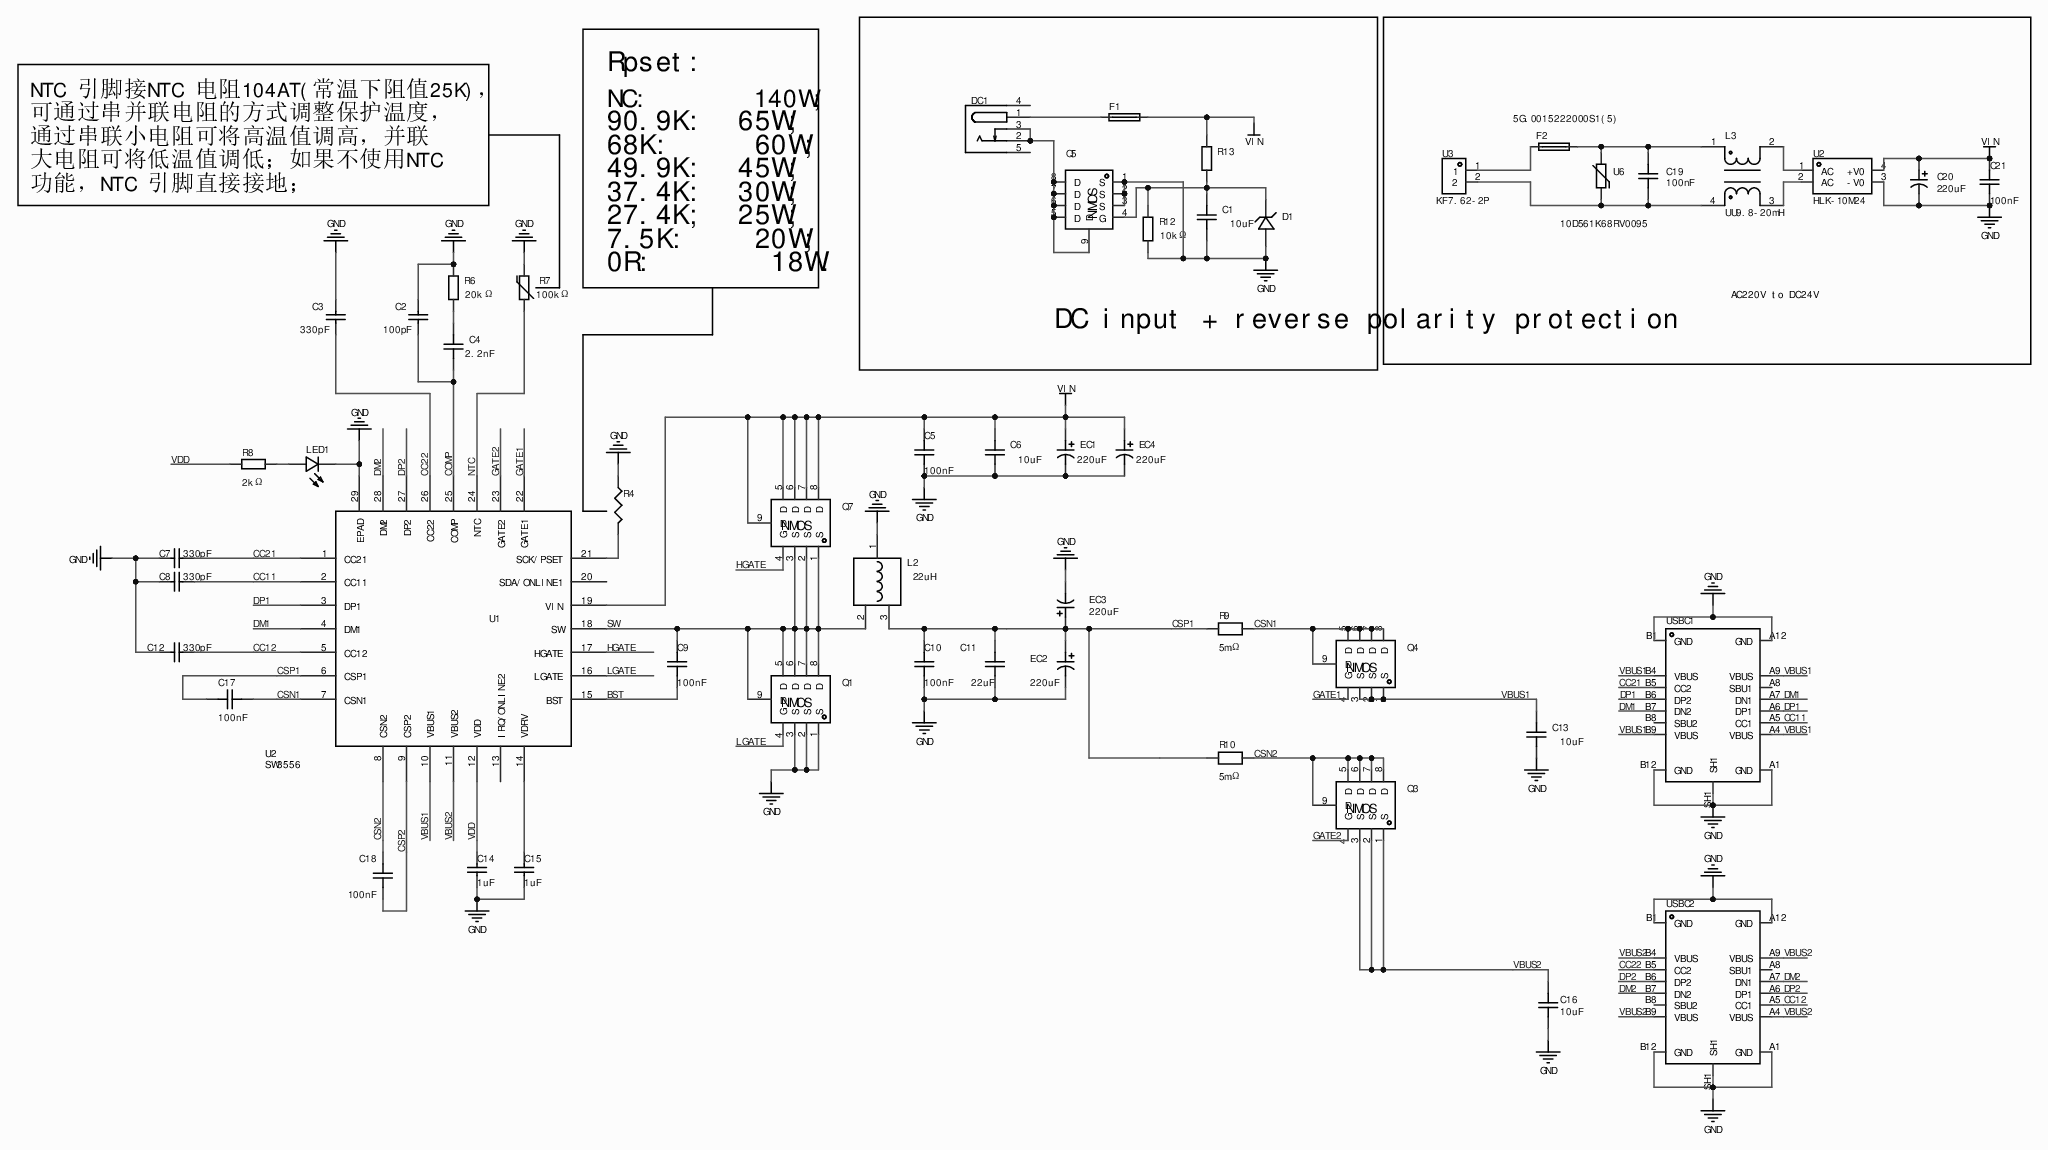
[diagram p0: MISC82101-2.schdoc]
# Altium project MISC82101-8.PrjPcb
1 sheet, 51 parts. Net scope: global (net labels, ports and power ports of the same name join across sheets).
Board file: MISC82101.pcbdoc

## Sheet MISC82101-2.schdoc
size 614 x 444 mm; @Project Name: MISC82101; @Page Count: 1; @Update Date: 2024-04-24; @Create Date: 2024-04-24; @Schematic Name: MISC82101; @Page No: 1

### Parts
C1  10uF  [C0805]
C2  100pF  [C0603]
C3  330pF  [C0603]
C4  2.2nF  [C0603]
C5  100nF  [C0603]
C6  10uF  [C0805]
C7  330pF  [C0603]
C8  330pF  [C0603]
C9  100nF  [C0603]
C10  100nF  [C0603]
C11  22uF  [C0805]
C12  330pF  [C0603]
C13  10uF  [C0805]
C14  1uF  [C0603]
C15  1uF  [C0603]
C16  10uF  [C0805]
C17  100nF  [C0603]
C18  100nF  [C0603]
C19  100nF  [CAP-TH_L13.0-W6.0-P10.0-D0.6]
C20  220uF  [CAP-TH_BD8.0-P3.50-D0.6-FD]
C21  100nF  [C0603]
D1  BZT52C3V3  [SOD-123_L2.7-W1.6-LS3.7-RD]  (value not drawn)
DC1  DC-044A-20A  [DC-IN-TH_DC-044A-20A]  (value not drawn)
EC1  220uF  [CAP-TH_BD8.0-P3.50-D0.6-FD-2]
EC2  220uF  [CAP-TH_BD8.0-P3.50-D0.6-FD-2]
EC3  220uF  [CAP-TH_BD8.0-P3.50-D0.6-FD-2]
EC4  220uF  [CAP-TH_BD8.0-P3.50-D0.6-FD-2]
F1  0451008.MRL  [FUSE-SMD_L6.1-W2.7]  (value not drawn)
F2  5G.0015222000S1(5)  [FUSE-TH_BD5.6-L21.0-P25.00-D0.7]
L2  22uH  [IND-SMD_3P-L15.5-W15.5-L]
L3  UU9.8-20mH  [FILTER-TH_4P-L17.0-W12.0-P7.00-D0.6-S8.00]
LED1  19-217/BHC-ZL1M2RY/3T  [LED0603-R-RD]  (value not drawn)
Q1  RUH4040M2  [PDFN3333-8_L3.1-W3.2-P0.65-LS3.4-BL]  (value not drawn)
Q3  RUH4040M2  [PDFN3333-8_L3.1-W3.2-P0.65-LS3.4-BL]  (value not drawn)
Q4  RUH4040M2  [PDFN3333-8_L3.1-W3.2-P0.65-LS3.4-BL]  (value not drawn)
Q5  RUH4040M2  [PDFN3333-8_L3.1-W3.2-P0.65-LS3.4-BL]  (value not drawn)
Q7  RUH4040M2  [PDFN3333-8_L3.1-W3.2-P0.65-LS3.4-BL]  (value not drawn)
R4  Rpset  [R0603]  (value not drawn)
R6  20kΩ  [R0603]
R7  Resistance @ 25℃: 100kΩ  [R0603]  (hidden comment: SDNT1608X104F4250FTF)
R8  value 2kΩ  [R0603]  (hidden comment: 0603WAF2001T5E)
R9  value 5mΩ  [R2010]  (hidden comment: RLM20FECR005)
R10  value 5mΩ  [R2010]  (hidden comment: RLM20FECR005)
R12  10kΩ  [R0603]
R13  0603WAF5102T5E  [R0603]  (value not drawn)
U1  sw3556-1  [QFN-28_L4.0-W4.0-P0.40-BL-EP]  (value not drawn)
U2  HLK-10M24  [PWRM-TH_HLK-10M24]
U3  KF7.62-2P  [CONN-TH_KF7.62-2P]
U6  10D561K68RV0095  [RES-TH_L13.5-W7.0-P7.50-S4.00-D0.7]
USBC1  U263-163N-4OS1735  [USB-C-SMD_U263-163N-4GS1735]  (value not drawn)
USBC2  U263-163N-4OS1735  [USB-C-SMD_U263-163N-4GS1735]  (value not drawn)

### Blocks framed on the sheet
DC input + reverse polarity protection: C1 D1 DC1 F1 Q5 R12 R13
AC220V to DC24V: C19-C21 F2 L3 U2 U3 U6

### Nets
GND: C1.1 C2.2 C3.2 C5.2 C6.1 C7.2 C8.2 C10.2 C11.1 C12.2 C13.1 C14.1 C15.1 C16.1 C20.2 C21.2 D1.2 EC1.2 EC2.2 EC3.2 EC4.2 L2.1 LED1.2(C) Q1.1(S) Q1.2(S) Q1.3(S) Q5.1(S) Q5.2(S) Q5.3(S) R4.1 R6.2 R7.1 R12.1 U1.29(EPAD) U2.3(-V0) USBC1.A1(GND) USBC1.A12(GND) USBC1.B1(GND) USBC1.B12(GND) USBC1.SH1 USBC2.A1(GND) USBC2.A12(GND) USBC2.B1(GND) USBC2.B12(GND) USBC2.SH1
VIN: C5.1 C6.2 C20.1 C21.1 EC1.1 EC4.1 F1.2 Q7.5(D) Q7.6(D) Q7.7(D) Q7.8(D) Q7.9(D) R13.2 U1.19(VIN) U2.4(+V0)
BST: C9.2 U1.15(BST)
CC11: C8.1 U1.2(CC11) USBC1.A5(CC1)
CC12: C12.1 U1.5(CC12) USBC2.A5(CC1)
CC21: C7.1 U1.1(CC21) USBC1.B5(CC2)
CC22: C3.1 U1.26(CC22) USBC2.B5(CC2)
COMP: C2.1 C4.1 U1.25(COMP)
CSN1: C17.1 Q4.5(D) Q4.6(D) Q4.7(D) Q4.8(D) Q4.9(D) R9.2 U1.7(CSN1)
CSN2: C18.1 Q3.5(D) Q3.6(D) Q3.7(D) Q3.8(D) Q3.9(D) R10.2 U1.8(CSN2)
CSP1: C10.1 C11.2 C17.2 C18.2 EC2.1 EC3.1 L2.3 R9.1 R10.1 U1.6(CSP1) U1.9(CSP2)  [also labelled CSP2, VOUT]
DM1: U1.4(DM1) USBC1.A7(DN1) USBC1.B7(DN2)
DM2: U1.28(DM2) USBC2.A7(DN1) USBC2.B7(DN2)
DP1: U1.3(DP1) USBC1.A6(DP1) USBC1.B6(DP2)
DP2: U1.27(DP2) USBC2.A6(DP1) USBC2.B6(DP2)
GATE1: Q4.4(G) U1.22(GATE1)
GATE2: Q3.4(G) U1.23(GATE2)
HGATE: Q7.4(G) U1.17(HGATE)
LGATE: Q1.4(G) U1.16(LGATE)
NTC: R7.2 U1.24(NTC)
SW: C9.1 L2.2 Q1.5(D) Q1.6(D) Q1.7(D) Q1.8(D) Q1.9(D) Q7.1(S) Q7.2(S) Q7.3(S) U1.18(SW)
VBUS1: C13.2 Q4.1(S) Q4.2(S) Q4.3(S) U1.10(VBUS1) USBC1.A4(VBUS) USBC1.A9(VBUS) USBC1.B4(VBUS) USBC1.B9(VBUS)
VBUS2: C16.2 Q3.1(S) Q3.2(S) Q3.3(S) U1.11(VBUS2) USBC2.A4(VBUS) USBC2.A9(VBUS) USBC2.B4(VBUS) USBC2.B9(VBUS)
VDD: C14.2 R8.1 U1.12(VDD)
NetC1_2: C1.2 D1.1 Q5.4(G) R12.2 R13.1
NetC4_2: C4.2 R6.1
NetC15_2: C15.2 U1.14(VDRV)
NetC19_1: C19.1 L3.4 U3.2 U6.1
NetC19_2: C19.2 F2.2 L3.1 U6.2
NetDC1_1: DC1.1 F1.1
NetDC1_2: DC1.2 DC1.3 Q5.5(D) Q5.6(D) Q5.7(D) Q5.8(D) Q5.9(D)
NetF2_1: F2.1 U3.1
NetL3_2: L3.2 U2.1(AC)
NetL3_3: L3.3 U2.2(AC)
NetLED1_1: LED1.1(A) R8.2
NetR4_2: R4.2 U1.21(SCK/PSET)

Not connected (* = marked no-connect by the designer): DC1 4* 5*; U1 13(IRQ/ONLINE2)* 20(SDA/ONLINE1)*; USBC1 A8(SBU1)* B8(SBU2)*; USBC2 A8(SBU1)* B8(SBU2)*

### Notes on the sheet
- Rpset:
- NC:       140W;
- 90.9K:  65W;
- 68K:     60W;
- 49.9K:  45W;
- NTC 引脚接NTC 电阻104AT(常温下阻值25K)，
  可通过串并联电阻的方式调整保护温度，
  通过串联小电阻可将高温值调高，并联
  大电阻可将低温值调低；如果不使用NTC
  功能，NTC 引脚直接接地；
- 37.4K:  30W;
- 27.4K;  25W;
- 7.5K:    20W;
- 0R:       18W.
- 1
- A

### Library data of the parts
C1 C6 C13 C16 = 10uF: Capacitance: 10uF; tolerance: ±10%; rated voltage: 50V; dielectric (temperature coefficient): X5R;; Manufacturer: muRata(村田); Symbol: GRM21BR61H106KE43L; Add into BOM: yes; Name: 10uF; Device: 10uF; LCSC Part Name: 10uF ±10% 50V; Supplier Part: C440198; Manufacturer Part: GRM21BR61H106KE43L; Supplier Footprint: 0805; JLCPCB Part Class: Basic library; Datasheet: https://atta.szlcsc.com/upload/public/pdf/source/20191220/C440198_2DEA1B9834E321C8893F7972E9DFE5B0.pdf; Supplier: LCSC; Convert to PCB: yes; Value: 10uF; Tolerance: ±10%; Voltage Rated: 50V; Temperature Coefficient: X5R; Origin Footprint 2: C0805; Origin Footprint 1: GRM21BR61H106KE43L
C2 = 100pF: Capacitance: 100pF; tolerance: ±5%; rated voltage: 50V; dielectric (temperature coefficient): C0G;; Manufacturer: SAMSUNG(三星); Symbol: CL10C101JB8NNNC; Add into BOM: yes; Name: 100pF; Device: 100pF; LCSC Part Name: 100pF ±5% 50V; Supplier Part: C14858; Manufacturer Part: CL10C101JB8NNNC; Supplier Footprint: 0603; JLCPCB Part Class: Basic library; Datasheet: https://atta.szlcsc.com/upload/public/pdf/source/20160103/1457707672333.pdf; Supplier: LCSC; Convert to PCB: yes; Value: 100pF; Tolerance: ±5%; Voltage Rated: 50V; Temperature Coefficient: C0G; Origin Footprint 2: C0603; Origin Footprint 1: CL10C101JB8NNNC
C3 C7 C8 C12 = 330pF: Capacitance: 330pF; tolerance: ±5%; rated voltage: 50V; dielectric (temperature coefficient): C0G;; Manufacturer: SAMSUNG(三星); Symbol: CL10C331JB8NNNC; Add into BOM: yes; Name: 330pF; Device: 330pF; LCSC Part Name: 330pF ±5% 50V; Supplier Part: C1664; Manufacturer Part: CL10C331JB8NNNC; Supplier Footprint: 0603; JLCPCB Part Class: Basic library; Datasheet: https://atta.szlcsc.com/upload/public/pdf/source/20160103/1457707688612.pdf; Supplier: LCSC; Convert to PCB: yes; Value: 330pF; Tolerance: ±5%; Voltage Rated: 50V; Temperature Coefficient: C0G; Origin Footprint 2: C0603; Origin Footprint 1: CL10C331JB8NNNC
C4 = 2.2nF: Capacitance: 2.2nF; tolerance: ±1%; rated voltage: -; dielectric (temperature coefficient): -;; Manufacturer: muRata(村田); Symbol: GCM1885C1H222FA16D; Add into BOM: yes; Name: 2.2nF; Device: 2.2nF; LCSC Part Name: 2.2nF ±1%; Supplier Part: C882578; Manufacturer Part: GCM1885C1H222FA16D; Supplier Footprint: 0603; JLCPCB Part Class: Extended library; Datasheet: https://atta.szlcsc.com/upload/public/pdf/source/20201228/C882578_EDF992AD6064A2D085B371C371799E69.pdf; Supplier: LCSC; Convert to PCB: yes; Value: 2.2nF; Tolerance: ±1%; Voltage Rated: -; Temperature Coefficient: -; Origin Footprint 2: C0603; Origin Footprint 1: GCM1885C1H222FA16D
C5 C9 C10 C17 C18 C21 = 100nF: Capacitance: 100nF; tolerance: ±10%; rated voltage: 50V; dielectric (temperature coefficient): X7R;; Manufacturer: YAGEO(国巨); Symbol: CC0603KRX7R9BB104; Add into BOM: yes; Name: 100nF; Device: 100nF; LCSC Part Name: 100nF ±10% 50V; Supplier Part: C14663; Manufacturer Part: CC0603KRX7R9BB104; Supplier Footprint: 0603; JLCPCB Part Class: Basic library; Datasheet: https://atta.szlcsc.com/upload/public/pdf/source/20170116/1484561234239.pdf; Supplier: LCSC; Convert to PCB: yes; Value: 100nF; Tolerance: ±10%; Voltage Rated: 50V; Temperature Coefficient: X7R; Origin Footprint 2: C0603; Origin Footprint 1: CC0603KRX7R9BB104
C11 = 22uF: Capacitance: 22uF; tolerance: ±20%; rated voltage: 25V; dielectric (temperature coefficient): X5R;; Manufacturer: SAMSUNG(三星); Manufacturer Part: CL21A226MAQNNNE; Symbol: CL21A226MAQNNNE_C45783; Add into BOM: yes; Name: 22uF; Device: 22uF; LCSC Part Name: 22uF ±20% 25V; Supplier Part: C45783; Supplier Footprint: 0805; JLCPCB Part Class: Basic library; Datasheet: https://atta.szlcsc.com/upload/public/pdf/source/20160103/1457707727161.pdf; Supplier: LCSC; Convert to PCB: yes; Value: 22uF; Tolerance: ±20%; Voltage Rated: 25V; Temperature Coefficient: X5R; Origin Footprint 2: C0805; Origin Footprint 1: CL21A226MAQNNNE_C45783
C14 C15 = 1uF: Capacitance: 1uF; tolerance: ±10%; rated voltage: 50V; dielectric (temperature coefficient): X5R;; Manufacturer: SAMSUNG(三星); Symbol: CL10A105KB8NNNC; Add into BOM: yes; Name: 1uF; Device: 1uF; LCSC Part Name: 1uF ±10% 50V; Supplier Part: C15849; Manufacturer Part: CL10A105KB8NNNC; Supplier Footprint: 0603; JLCPCB Part Class: Basic library; Datasheet: https://atta.szlcsc.com/upload/public/pdf/source/20160103/1457707679084.pdf; Supplier: LCSC; Convert to PCB: yes; Value: 1uF; Tolerance: ±10%; Voltage Rated: 50V; Temperature Coefficient: X5R; Origin Footprint 2: C0603; Origin Footprint 1: CL10A105KB8NNNC
C19 = X2-104K-275VAC_C914483: Manufacturer: NDF(达孚); Add into BOM: yes; Tolerance: ±10%; Voltage(AC): 275V; Subclass: X2; Name: 100nF; Symbol: X2-104K-275VAC_C914483; Device: X2-104K-275VAC_C914483; LCSC Part Name: 等级:X2 100nF ±10% 275V; Supplier Part: C914483; Manufacturer Part: X2-104K-275VAC; Supplier Footprint: 插件,P=10mm; JLCPCB Part Class: Extended library; Datasheet: https://atta.szlcsc.com/upload/public/pdf/source/20210517/C914484_87B6324D9C831D7B5ED24756D36395BD.pdf; Supplier: LCSC; Convert to PCB: yes; Value: 100nF; Operating Temperature: -40℃~+110℃
C20 = 01EC3470: Manufacturer: KNSCHA(科尼盛); Add into BOM: yes; Tolerance: ±20%; Rated Voltage: 50V; Ripple Current: 350mA@120kHz; φD: 8mm; L: 12mm; Lifetime @ Temp: 2000hrs@105℃; Name: 220uF; Symbol: 01EC3470; Device: 01EC3470; Supplier: LCSC; Supplier Part: C2836445; Manufacturer Part: 01EC3470; Value: 220uF; JLCPCB Part Class: Extended library; LCSC Part Name: 220uF ±20% 50V; Supplier Footprint: 插件,D8xL12mm; Datasheet: https://atta.szlcsc.com/upload/public/pdf/source/20210528/C2836445_4EB3DEC3C45633977FB5495C9B2E1697.pdf; Convert to PCB: yes; Equivalent Series Resistance(ESR): -; Lead Spacing: 3.5mm; Operating Temperature: -40℃~+105℃
D1 = BZT52C3V3: Diode configuration: single; zener voltage (nominal): 3.3V; zener voltage (range): 3.1V~3.5V; tolerance: ±5%; power: 500mW; reverse current (Ir): 20uA@1V; impedance (Zzt): 130Ω;; Manufacturer: SHIKUES(时科); Symbol: BZT52C3V3_C216707; Add into BOM: yes; Name: BZT52C3V3; Device: BZT52C3V3; LCSC Part Name: 3.3V ±5% 500mW; Supplier Part: C216707; Manufacturer Part: BZT52C3V3; Supplier Footprint: SOD-123; JLCPCB Part Class: Extended library; Datasheet: https://atta.szlcsc.com/upload/public/pdf/source/20180516/C216707_F0EE676A8DB3508FCF1A2E5208384022.pdf; Supplier: LCSC; Convert to PCB: yes; Diode Configuration: Single; Zener Voltage (Nom): 3.3V; Zener Voltage (Range): 3.1V~3.5V; Tolerance: ±5%; Power Dissipation: 500mW; Reverse Leakage Current (Ir): 20uA@1V; Zener Impedance (Zzt): 130Ω; Origin Footprint 2: SOD-123_L2.7-W1.6-LS3.7-RD; Origin Footprint 1: BZT52C3V3_C216707
DC1 = DC-044A-20A: Contact inner diameter: 2mm; contact outer diameter: 5.9mm; rated current: 500mA; rated voltage: 30V;; Manufacturer: 韩国韩荣; Add into BOM: yes; Name: DC-044A-20A; Symbol: DC-044A-20A; Device: DC-044A-20A; LCSC Part Name: 内径:2mm 外径:5.9mm; Supplier Part: C129006; Manufacturer Part: DC-044A-20A; Supplier Footprint: 插件; JLCPCB Part Class: Extended library; Datasheet: https://atta.szlcsc.com/upload/public/pdf/source/20210810/C8974B0AB7FDF70EB0A74D74746E6460.pdf; Supplier: LCSC; Convert to PCB: yes; Inside Contact Diameter: 2mm; Outside Contact Diameter: 5.9mm; Current Rating (Max): 500mA; Voltage Rating (Max): 30V; Origin Footprint 2: DC-IN-TH_DC-044A-20A; Origin Footprint 1: DC-044A-20A
EC1-EC4 = 220uF: 容值:220uF;精度:±20%;额定电压:35V;电容体直径:8mm;电容体长度:9mm;脚间距:3.5mm;纹波电流:1.7A@100kHz;等效串联电阻:40mΩ@100kHz;工作寿命:2000hrs@105℃;工作温度:-55℃~+105℃;; Manufacturer: KNSCHA(科尼盛); Symbol: KNH2220UF35V149EC0049; Add into BOM: yes; Tolerance: ±20%; Rated Voltage: 35V; φD: 8mm; L: 9mm; Name: 220uF; Device: 220uF; LCSC Part Name: 220uF ±20% 35V; Supplier Part: C2981462; Manufacturer Part: KNH2220UF35V149EC0049; Supplier Footprint: 径向引线,8x9mm; JLCPCB Part Class: Extended Part; Datasheet: https://atta.szlcsc.com/upload/public/pdf/source/20220426/9FC8A158D93B909CC105160B4A0CB698.pdf; Supplier: LCSC; Convert to PCB: yes; Value: 220uF; Lead Spacing: 3.5mm; Ripple Current: 1.7A@100kHz; Equivalent Series Resistance(ESR): 40mΩ@100kHz; Lifetime @ Temp: 2000hrs@105℃; Operating Temperature: -55℃~+105℃; Origin Footprint 2: CAP-TH_BD8.0-P3.50-D0.6-FD-2; Origin Footprint 1: KNH2220UF35V149EC0049
F1 = 0451008.MRL: Type: SMD fuse; rated current: 8A; rated voltage (AC): 125V; rated voltage (DC): 125V; breaking capacity: 50A; operating temperature: -55℃~+125℃;; Manufacturer: Littelfuse(美国力特); Add into BOM: yes; Name: 0451008.MRL; Symbol: 0451008.MRL; Device: 0451008.MRL; LCSC Part Name: 125VAC 8A 快断; Supplier Part: C142876; Manufacturer Part: 0451008.MRL; Supplier Footprint: SMD; JLCPCB Part Class: Extended library; Datasheet: https://atta.szlcsc.com/upload/public/pdf/source/20171109/C142876_15102200338961103550.pdf; Supplier: LCSC; Convert to PCB: yes; Current Rating: 8A; Voltage Rating  (AC): 125V; Voltage Rating (DC): 125V; Breaking Capacity: 50A; Operating Temperature: -55℃~+125℃; Origin Footprint 2: FUSE-SMD_L6.1-W2.7; Origin Footprint 1: 0451008.MRL
F2 = 5G.0015222000S1(5): Manufacturer: xcfuse(旭程); Add into BOM: yes; Type: Glass tube fuse; Current Rating: 15A; Name: 5G.0015222000S1(5); Symbol: 5G.0015222000S1(5); Device: 5G.0015222000S1(5); Supplier: LCSC; Supplier Part: C140517; Manufacturer Part: 5G.0015222000S1(5); JLCPCB Part Class: Extended library; LCSC Part Name: 玻璃管保险丝; Supplier Footprint: 插件,5.6x21mm; Datasheet: https://atta.szlcsc.com/upload/public/pdf/source/20180621/C140517_9B97A8C42A8CF3E19442F8E07BBBAF3C.pdf; Convert to PCB: yes
L2 = 22uH: Inductance: 22uH; tolerance: ±20%; rated current: 7.5A; DC resistance (DCR): 14.5mΩ;; Manufacturer: Sumida(胜美达); Symbol: CDEP15D90T150NP-220MC-125; Add into BOM: yes; Name: 22uH; Device: 22uH; LCSC Part Name: 22uH ±20% 7.5A 14.5mΩ; Supplier Part: C171581; Manufacturer Part: CDEP15D90T150NP-220MC-125; Supplier Footprint: SMD; JLCPCB Part Class: Extended library; Datasheet: https://atta.szlcsc.com/upload/public/pdf/source/20180612/C171581_D70A455BA7744A0B5218E235967B6B52.pdf; Supplier: LCSC; Convert to PCB: yes; Value: 22uH; Tolerance: ±20%; Rated Current: 7.5A; DC Resistance (DCR): 14.5mΩ; Origin Footprint 2: IND-SMD_3P-L15.5-W15.5-L; Origin Footprint 1: CDEP15D90T150NP-220MC-125
L3 = UU9.8-20mH: Manufacturer: FH(风华); Add into BOM: yes; Number of Lines: 2; Withstanding Voltage: 500V@1Mins; Inductance @ Frequency: 20mH@1kHz; DC Resistance (DCR): 3Ω; Name: UU9.8-20mH; Symbol: UU9.8-20MH; Device: UU9.8-20mH; LCSC Part Name: 两路 插件共模滤波器; Supplier Part: C164623; Manufacturer Part: UU9.8-20mH; Supplier Footprint: 插件; JLCPCB Part Class: Extended library; Datasheet: https://atta.szlcsc.com/upload/public/pdf/source/20180207/C164623_15179949983281359206.pdf; Supplier: LCSC; Convert to PCB: yes
LED1 = 19-217/BHC-ZL1M2RY/3T: Illumination color: blue; dominant wavelength / chromaticity: 465~475nm;; Manufacturer: EVERLIGHT(亿光); Add into BOM: yes; Luminous Intensity (IF=20mA): 11.5~28.5mcd@5mA; Origin Footprint 2: LED0603-R-RD_BLUE; Name: 19-217/BHC-ZL1M2RY/3T; Symbol: 19-217/BHC-ZL1M2RY/3T; Device: 19-217/BHC-ZL1M2RY/3T; LCSC Part Name: 0603 蓝灯; Supplier Part: C72041; Manufacturer Part: 19-217/BHC-ZL1M2RY/3T; Supplier Footprint: 0603; JLCPCB Part Class: Basic library; Datasheet: https://atta.szlcsc.com/upload/public/pdf/source/20170116/1484561237273.pdf; Supplier: LCSC; Convert to PCB: yes; Mounting Type: Surface mount; Illumination Color: Blue; Dominant Wavelength / Coordinate rank: 465~475nm; Origin Footprint 1: 19-217/BHC-ZL1M2RY/3T
Q1 Q3-Q5 Q7 = RUH4040M2: 类型:-;漏源电压(Vdss):-;连续漏极电流(Id):-;功率(Pd):-;导通电阻(RDS(on)@Vgs,Id):-;阈值电压(Vgs(th)@Id):-;栅极电荷(Qg@Vgs):-;输入电容(Ciss@Vds):-;反向传输电容(Crss@Vds):-;; Manufacturer: Ruichips(锐骏半导体); Add into BOM: yes; Name: RUH4040M2; Symbol: RUH4040M2; Device: RUH4040M2; LCSC Part Name: RUH4040M2; Supplier Part: C521556; Manufacturer Part: RUH4040M2; Supplier Footprint: PDFN3333; JLCPCB Part Class: Extended library; Datasheet: https://atta.szlcsc.com/upload/public/pdf/source/20200428/C521556_1F7C9517B2F2105A4BFBCF64B414A92D.pdf; Supplier: LCSC; Convert to PCB: yes; Type: -; Drain Source Voltage (Vdss): -; Continuous Drain Current (Id): -; Power Dissipation (Pd): -; Drain Source On Resistance (RDS(on)@Vgs,Id): -; Gate Threshold Voltage (Vgs(th)@Id): -; Total Gate Charge (Qg@Vgs): -; Input Capacitance (Ciss@Vds): -; Reverse Transfer Capacitance (Crss@Vds): -; Origin Footprint 2: PDFN3333-8_L3.1-W3.2-P0.65-LS3.4-BL; Origin Footprint 1: RUH4040M2
R4 = Rpset: Resistor; Symbol: 68K; Value: 2K; Origin Footprint 3: R0805; Origin Footprint 4: R1206; Origin Footprint 5: R2512; Add into BOM: yes; Name: Rpset; Device: Rpset; Published: 8-Jun-2000; LatestRevisionDate: 29-May-2009; LatestRevisionNote: IPC-7351 Footprint Added.; PackageReference: J1-0603; PackageDescription: Chip Resistor; Origin Footprint 2: R0603; Convert to PCB: yes; Origin Footprint 1: R0603; Design Item ID: RES; Library Name: Integrated library; Publisher: Altium Limited
R6 = 20kΩ: Tolerance: ±1%; temperature coefficient: ±100ppm/℃; resistance: 20kΩ; power: 1/10W; max working voltage: 75V; operating temperature range: -55℃~+155℃;; Manufacturer: UNI-ROYAL(厚声); Symbol: 0603WAF2002T5E; Add into BOM: yes; Name: 20kΩ; Device: 20kΩ; LCSC Part Name: 20KΩ ±1%; Supplier Part: C4184; Manufacturer Part: 0603WAF2002T5E; Supplier Footprint: 0603; JLCPCB Part Class: Basic library; Datasheet: https://atta.szlcsc.com/upload/public/pdf/source/20170920/C4184_1505887495503980652.pdf; Supplier: LCSC; Convert to PCB: yes; Temperature Coefficient: ±100ppm/℃; Value: 20kΩ; Power(Watts): 1/10W; Overload Voltage (Max): 75V; Operating Temperature Range: -55℃~+155℃; Origin Footprint 2: R0603; Origin Footprint 1: 0603WAF2002T5E
R7 = SDNT1608X104F4250FTF: 阻值(25℃):100kΩ;电阻精度:±1%;B值精度:±1%;B值(25℃/50℃):4250K;功率:100mW;最大稳态电流(25℃):100uA;B值(25℃/75℃):-;B值(25℃/85℃):-;B值(25℃/100℃):-;工作温度:-55℃~+125℃;; Manufacturer: Sunlord(顺络); Add into BOM: yes; Resistance Tolerance: ±1%; B Constant (25℃/50℃): 4250K; Power: 100mW; Steady State Current (Max): 100uA; Name: SDNT1608X104F4250FTF; Symbol: SDNT1608X104F4250FTF; Device: SDNT1608X104F4250FTF; LCSC Part Name: 100kΩ 电阻精度:±1% 4250K; Supplier Part: C95955; Manufacturer Part: SDNT1608X104F4250FTF; Supplier Footprint: 0603; JLCPCB Part Class: Extended library; Datasheet: https://atta.szlcsc.com/upload/public/pdf/source/20210916/BF106A3565EDFEB141CB3E0EA3A661F8.pdf; Supplier: LCSC; Convert to PCB: yes; B Constant Tolerance: ±1%; B Constant (25℃/75℃): -; B Constant (25℃/85℃): -; B Constant (25℃/100℃): -; Operating Temperature: -55℃~+125℃; Origin Footprint 2: R0603; Origin Footprint 1: SDNT1608X104F4250FTF
R8 = 0603WAF2001T5E: Tolerance: ±1%; resistance: 2kΩ; temperature coefficient: ±100ppm/℃; power: 1/10W; max working voltage: 75V; operating temperature range: -55℃~+155℃;; Manufacturer: UNI-ROYAL(厚声); Add into BOM: yes; Name: 0603WAF2001T5E; Symbol: 0603WAF2001T5E; Device: 0603WAF2001T5E; LCSC Part Name: 2KΩ ±1%; Supplier Part: C22975; Manufacturer Part: 0603WAF2001T5E; Supplier Footprint: 0603; JLCPCB Part Class: Basic library; Datasheet: https://atta.szlcsc.com/upload/public/pdf/source/20170920/C22975_1505901012894982362.pdf; Supplier: LCSC; Convert to PCB: yes; Temperature Coefficient: ±100ppm/℃; Power(Watts): 1/10W; Overload Voltage (Max): 75V; Operating Temperature Range: -55℃~+155℃; Origin Footprint 2: R0603; Origin Footprint 1: 0603WAF2001T5E
R9 R10 = RLM20FECR005: Resistor type: sense resistor; rated current: -; rated voltage drop: -; resistance: 5mΩ; tolerance: ±1%; power: 1W; temperature coefficient: ±50ppm/℃; mounting: SMD;; Manufacturer: 大毅科技; Add into BOM: yes; Name: RLM20FECR005; Symbol: RLM20FECR005; Device: RLM20FECR005; LCSC Part Name: 5mΩ ±1% 1W; Supplier Part: C912935; Manufacturer Part: RLM20FECR005; Supplier Footprint: 2010; JLCPCB Part Class: Extended library; Datasheet: https://atta.szlcsc.com/upload/public/pdf/source/20200810/C393093_263C75BBADC7FA82F8FCFD62085F9B59.pdf; Supplier: LCSC; Convert to PCB: yes; Type: Sense resistor; Rated Current: -; Rated Output Voltage: -; Tolerance: ±1%; Power(Watts): 1W; Temperature Coefficient: ±50ppm/℃; Mounting Sytle: SMD; Origin Footprint 2: R2010; Origin Footprint 1: RLM20FECR005
R12 = 10kΩ: Resistor type: thick film; resistance: 10kΩ; tolerance: ±1%; power: 100mW; temperature coefficient: ±100ppm/℃; max working voltage: 75V; operating temperature range: -55℃~+155℃;; Manufacturer: UNI-ROYAL(厚声); Symbol: 0603WAF1002T5E; Add into BOM: yes; Name: 10kΩ; Device: 10kΩ; LCSC Part Name: 10kΩ ±1% 100mW; Supplier Part: C25804; Manufacturer Part: 0603WAF1002T5E; Supplier Footprint: 0603; JLCPCB Part Class: Basic library; Datasheet: https://atta.szlcsc.com/upload/public/pdf/source/20200306/C422600_1E6D84923E4A46A82E41ADD87F860B5C.pdf; Supplier: LCSC; Convert to PCB: yes; Type: Thick film resistor; Value: 10kΩ; Tolerance: ±1%; Power(Watts): 100mW; Temperature Coefficient: ±100ppm/℃; Overload Voltage (Max): 75V; Operating Temperature Range: -55℃~+155℃; Origin Footprint 2: R0603; Origin Footprint 1: 0603WAF1002T5E
R13 = 0603WAF5102T5E: Manufacturer: UNI-ROYAL(厚声); Add into BOM: yes; Name: 0603WAF5102T5E; Symbol: 0603WAF5102T5E; Device: 0603WAF5102T5E; LCSC Part Name: 51KΩ(5102) ±1% 编带; Supplier Part: C23196; Manufacturer Part: 0603WAF5102T5E; Supplier Footprint: 0603; JLCPCB Part Class: Basic library; Datasheet: https://atta.szlcsc.com/upload/public/pdf/source/20170920/C23196_1505901126822982578.pdf; Supplier: LCSC; Convert to PCB: yes; Origin Footprint 2: R0603; Origin Footprint 1: 0603WAF5102T5E
U1 = sw3556-1: Add into BOM: yes; Name: sw3556-1; Symbol: sw3556-1; Device: sw3556-1; Convert to PCB: yes; Origin Footprint 2: QFN-28_L4.0-W4.0-P0.40-BL-EP; Origin Footprint 1: sw3556-1
U2 = HLK-10M24: Manufacturer: HI-LINK(海凌科); Add into BOM: yes; Conversion Type: AC-DC; Output Voltage: 24V; Output Power: 10W; Input Voltage(AC): 85VAC~265VAC; Output Current (Max): 420mA; Function: Step-down; Output Channel: 1; Insulated Voltage: 3kV@AC; Conversion Efficiency: 80%; Name: HLK-10M24; Symbol: HLK-10M24; Device: HLK-10M24; LCSC Part Name: HLK-10M24; Supplier Part: C2941419; Manufacturer Part: HLK-10M24; Supplier Footprint: DIP-4; JLCPCB Part Class: Extended library; Datasheet: https://atta.szlcsc.com/upload/public/pdf/source/20230506/347354FD6825E03F8DF380E9A4C93618.pdf; Supplier: LCSC; Convert to PCB: yes
U3 = KF7.62-2P: Manufacturer: KEFA(科发); Add into BOM: yes; Barrier Type: Dual row; Pitch: 7.62mm; Structure: 1x2P; Pin Location: Side pins; Current Rating (Max): 24A; Voltage Rating (Max): 450V; Wire Gauge - AWG: 12~22; Wire Gauge - mm2: 2.5; Number of PINs Per Row: 2; Name: KF7.62-2P; Symbol: KF7.62-2P; Device: KF7.62-2P; LCSC Part Name: 7.62mm 1x2P 每排P数:2 排数:1 直针 边脚 黑色; Supplier Part: C707824; Manufacturer Part: KF7.62-2P; Supplier Footprint: 插件,P=7.62mm; JLCPCB Part Class: Extended library; Datasheet: https://atta.szlcsc.com/upload/public/pdf/source/20230331/11104CA872B730518BFDFC9F574D6E42.pdf; Supplier: LCSC; Convert to PCB: yes; Mounting Style: Straight pin; Number of Pins: 2P; Number of Rows: 1; Operating Temperature Range: -40℃~+105℃; Color: Black
U6 = 10D561K68RV0095: Manufacturer: KNSCHA(科尼盛); Add into BOM: yes; Varistor Voltage: 504V~616V; Clamping Voltage: 920V; Allowable Voltage (DC): 460V; Allowable Voltage (AC): 350V; Peak Current: 1.25kA; Maximum Energy: 49J; Typical Capatitance: 180pF@1kHz; Name: 10D561K68RV0095; Symbol: 10D561K68RV0095; Device: 10D561K68RV0095; Supplier: LCSC; Supplier Part: C2840665; Manufacturer Part: 10D561K68RV0095; LCSC Part Name: 钳位电压920V 49焦耳 插件压敏电阻; Supplier Footprint: 插件,P=7.5mm; JLCPCB Part Class: Extended Part; Datasheet: https://atta.szlcsc.com/upload/public/pdf/source/20210618/C2840665_DBBEB4F695FE16B1EEDA4486CE1D1922.pdf; Convert to PCB: yes
USBC1 USBC2 = U263-163N-4OS1735: 连接器类型:Type-C;标准:USB 3.1;公母:母座;触点数量:16;端口数量:1;安装方式:卧贴;额定电流 - 电源:5A;触头材质:铜合金;触头镀层:金;工作温度范围:-25℃~+85℃;焊接温度(最大值):260℃;; Manufacturer: XKB Connectivity(中国星坤); Add into BOM: yes; Connector Type: Type-C; Gender: Female; Number of Contacts: 16; Number of Ports: 1; Current Rating - Power (Max): 5A; Welding Temperature (Max): 260℃; Name: U263-163N-4OS1735; Symbol: U263-163N-4OS1735; Device: U263-163N-4OS1735; LCSC Part Name: Type-C 母座 卧贴; Supplier Part: C2931472; Manufacturer Part: U263-163N-4OS1735; Supplier Footprint: SMD; JLCPCB Part Class: Extended library; Datasheet: https://atta.szlcsc.com/upload/public/pdf/source/20211215/D777AAC9FA67A227A25094451B68E75F.pdf; Supplier: LCSC; Convert to PCB: yes; Standard: USB 3.1; Mounting Style: Horizontal mount; Contact Material: Copper alloy; Contact Plating: Gold; Operating Temperature Range: -25℃~+85℃; Origin Footprint 2: USB-C-SMD_U263-163N-4GS1735; Origin Footprint 1: U263-163N-4OS1735